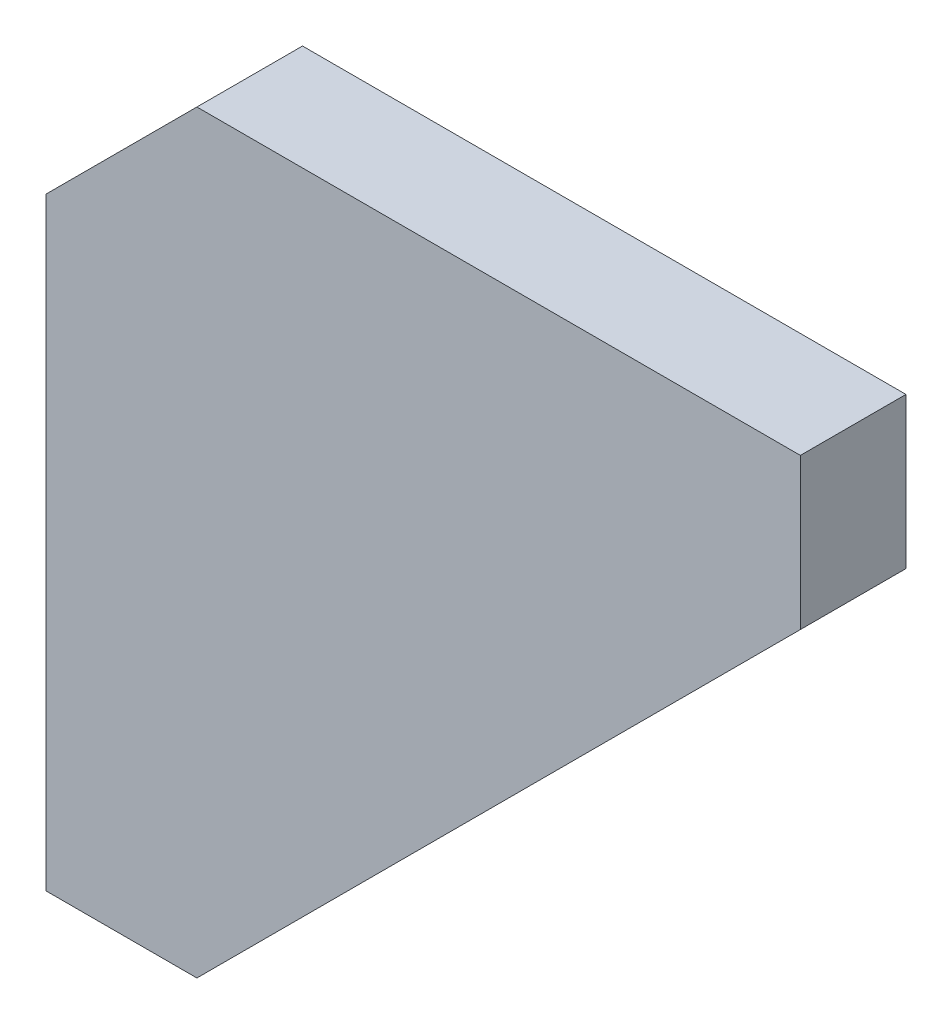
from build123d import *

# Parameters (mm, degrees)
EXTRUDE_1_DEPTH = 14


with BuildPart() as part:
    # 草图1 → 凸台-拉伸1 (new body)
    with BuildSketch(Plane.XY):
        Polygon((0, 0), (20, 0), (100, 80), (100, 100), (20, 100), (0, 80), align=None)
    extrude(amount=EXTRUDE_1_DEPTH)


solid = part.part
